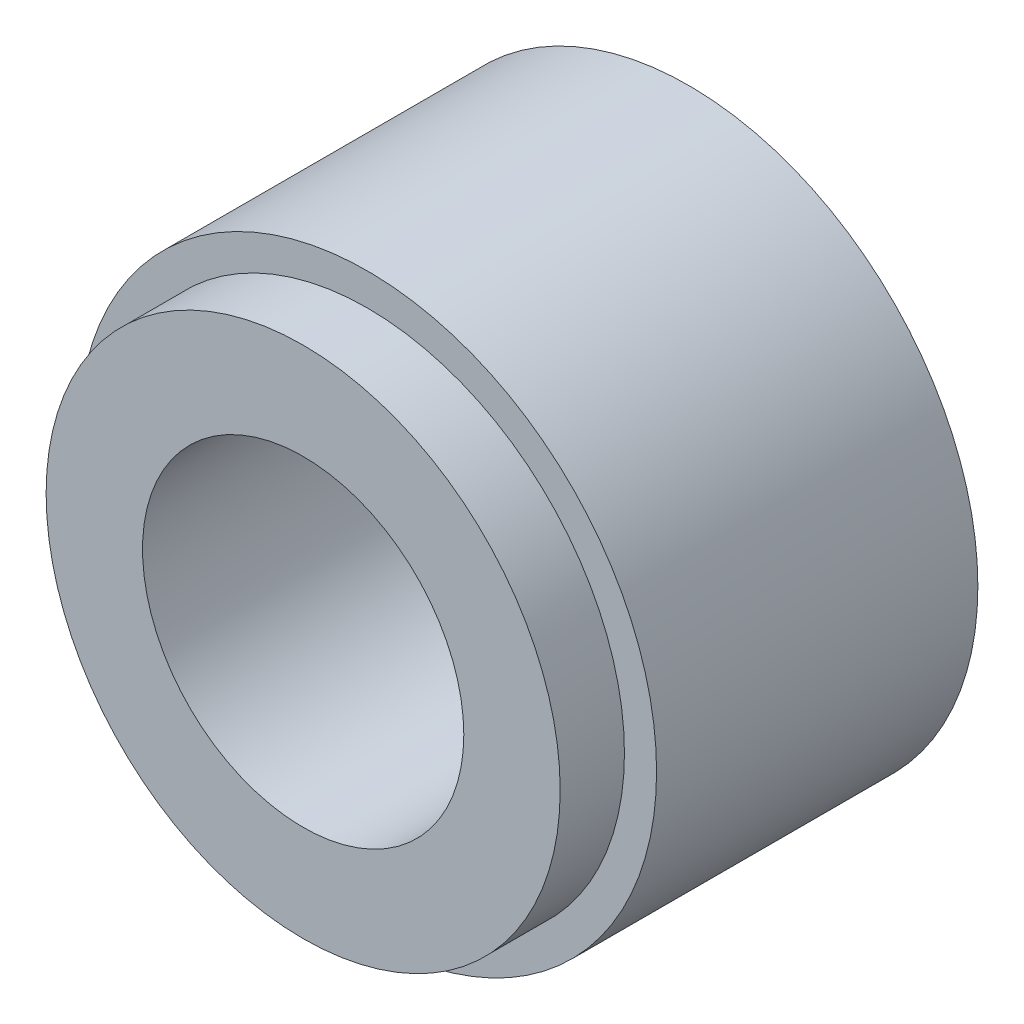
SolidWorks part; units mm, degrees
ref_plane "前视" through (0, 0, 0) normal (0, 0, 1) x (1, 0, 0)
ref_plane "上视" through (0, 0, 0) normal (0, 1, 0) x (1, 0, 0)
ref_plane "右视" through (0, 0, 0) normal (1, 0, 0) x (0, 0, -1)
sketch "草图1" plane through (0, 0, 0) normal (0, 0, 1) x (1, 0, 0)
  circle A0 centre (0, 0) radius 4.5
  circle A1 centre (0, 0) radius 2.5
extrude "凸台-拉伸1" add sketch "草图1" along normal blind 5
sketch "草图2" plane through (0, 0, 5) normal (0, 0, 1) x (1, 0, 0)
  circle A0 centre (0, 0) radius 2.5
  circle A1 centre (0, 0) radius 4
extrude "凸台-拉伸2" add sketch "草图2" along normal blind 1
